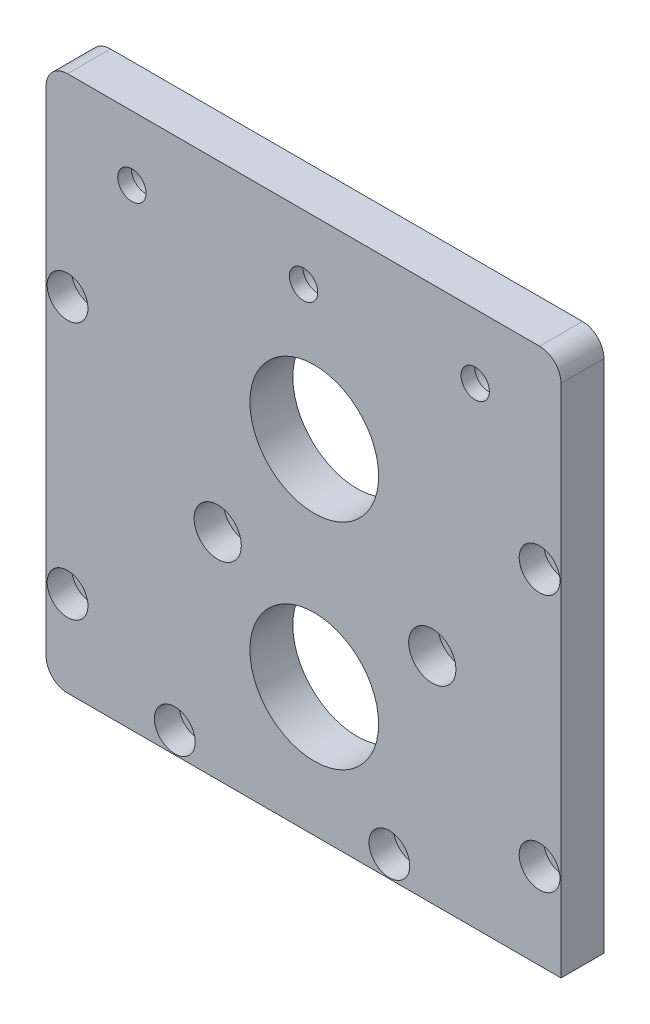
from build123d import *

# Parameters (mm, degrees)
SKETCH_1_W                = 120
SKETCH_1_H                = 220
EXTRUDE_1_DEPTH           = 10
HOLE_WIZARD_2_D           = 5.5
HOLE_WIZARD_2_CBORE_D     = 9.5
HOLE_WIZARD_2_CBORE_DEPTH = 5.7
HOLE_WIZARD_3_D           = 6.6
HOLE_WIZARD_3_CBORE_D     = 11
HOLE_WIZARD_3_CBORE_DEPTH = 6.8
FILLET_1_R                = 5
CUT_EXTRUDE_1_REACH       = 127.698
SKETCH_11_W               = 120
SKETCH_11_H               = 95
HOLE_WIZARD_4_D           = 6.6
HOLE_WIZARD_4_CBORE_D     = 11
HOLE_WIZARD_4_CBORE_DEPTH = 6.8
FILLET_2_R                = 5
CUT_EXTRUDE_2_REACH       = 127.698
SKETCH_14_R               = 15
HOLE_WIZARD_5_D           = 5.5
HOLE_WIZARD_5_DEPTH       = 20.4
HOLE_WIZARD_5_CBORE_D     = 9.5
HOLE_WIZARD_5_CBORE_DEPTH = 5.7
HOLE_WIZARD_5_TIP         = 1.652366702


with BuildPart() as part:
    # 草图1 → 凸台-拉伸1 (new body)
    with BuildSketch(Plane.XY):
        Rectangle(SKETCH_1_W, SKETCH_1_H)
    extrude(amount=EXTRUDE_1_DEPTH)

    # 打孔尺寸(%根据)内六角圆柱头螺钉的类型2 (through all)
    with Locations(Plane.XY.offset(10)):
        with Locations((-55, -30), (-55, -90)):
            hole_wizard_2 = CounterBoreHole(HOLE_WIZARD_2_D / 2, HOLE_WIZARD_2_CBORE_D / 2, HOLE_WIZARD_2_CBORE_DEPTH)

    # 打孔尺寸(%根据)内六角圆柱头螺钉的类型3 (through all)
    with Locations(Plane.XY.offset(10)):
        with Locations((-20, -60), (30, -60)):
            CounterBoreHole(HOLE_WIZARD_3_D / 2, HOLE_WIZARD_3_CBORE_D / 2, HOLE_WIZARD_3_CBORE_DEPTH)

    # 圆角1
    fillet_1_edges = [part.edges().sort_by_distance(p)[0] for p in [
        (-60, 110, 5),
        (-60, -110, 5),
    ]]
    fillet(fillet_1_edges, radius=FILLET_1_R)

    # 草图11 → 切除-拉伸1 (cut, up to next)
    with BuildSketch(Plane(origin=(0, 0, 0), x_dir=(-1, 0, 0), z_dir=(0, 0, -1)), mode=Mode.PRIVATE) as cut_extrude_1_sk1:
        with Locations((0, 62.5)):
            Rectangle(SKETCH_11_W, SKETCH_11_H)
    cut_extrude_1_tool1 = extrude(cut_extrude_1_sk1.sketch, amount=-CUT_EXTRUDE_1_REACH, mode=Mode.PRIVATE) & part.part
    add(cut_extrude_1_tool1.solids().sort_by_distance((0, 62.5, 0))[0], mode=Mode.SUBTRACT)

    # 打孔尺寸(%根据)内六角圆柱头螺钉的类型4 (through all)
    with Locations(Plane(origin=(0, 0, 0), x_dir=(-1, 0, 0), z_dir=(0, 0, -1))):
        with Locations((-40, 0), (0, 0), (40, 0)):
            CounterBoreHole(HOLE_WIZARD_4_D / 2, HOLE_WIZARD_4_CBORE_D / 2, HOLE_WIZARD_4_CBORE_DEPTH)

    # 圆角2
    fillet_2_edges = [part.edges().sort_by_distance(p)[0] for p in [
        (60, 15, 5),
        (-60, 15, 5),
    ]]
    fillet(fillet_2_edges, radius=FILLET_2_R)

    # 草图14 → 切除-拉伸2 (cut, up to next)
    with BuildSketch(Plane(origin=(0, 0, 0), x_dir=(-1, 0, 0), z_dir=(0, 0, -1)), mode=Mode.PRIVATE) as cut_extrude_2_sk1:
        with Locations((-2.5, -30)):
            Circle(SKETCH_14_R)
    cut_extrude_2_tool1 = extrude(cut_extrude_2_sk1.sketch, amount=-CUT_EXTRUDE_2_REACH, mode=Mode.PRIVATE) & part.part
    # 草图14 → 切除-拉伸2 (cut, up to next)
    with BuildSketch(Plane(origin=(0, 0, 0), x_dir=(-1, 0, 0), z_dir=(0, 0, -1)), mode=Mode.PRIVATE) as cut_extrude_2_sk2:
        with Locations((-2.5, -80)):
            Circle(SKETCH_14_R)
    cut_extrude_2_tool2 = extrude(cut_extrude_2_sk2.sketch, amount=-CUT_EXTRUDE_2_REACH, mode=Mode.PRIVATE) & part.part
    add(cut_extrude_2_tool1.solids().sort_by_distance((2.5, -30, 0))[0], mode=Mode.SUBTRACT)
    add(cut_extrude_2_tool2.solids().sort_by_distance((2.5, -80, 0))[0], mode=Mode.SUBTRACT)

    # 镜向1: 打孔尺寸(%根据)内六角圆柱头螺钉的类型2 across plane
    add(hole_wizard_2.mirror(Plane(origin=(0, 0, 0), x_dir=(0, 0, 1), z_dir=(1, 0, 0))), mode=Mode.SUBTRACT)

    # 打孔尺寸(%根据)内六角圆柱头螺钉的类型5
    with Locations(Plane.XY.offset(10)):
        with Locations((20, -105), (-30, -105)):
            CounterBoreHole(HOLE_WIZARD_5_D / 2, HOLE_WIZARD_5_CBORE_D / 2, HOLE_WIZARD_5_CBORE_DEPTH, depth=HOLE_WIZARD_5_DEPTH)
            with Locations((0, 0, -(HOLE_WIZARD_5_DEPTH + HOLE_WIZARD_5_TIP / 2))):  # 118° drill point
                Cone(0, HOLE_WIZARD_5_D / 2, HOLE_WIZARD_5_TIP, mode=Mode.SUBTRACT)


solid = part.part
